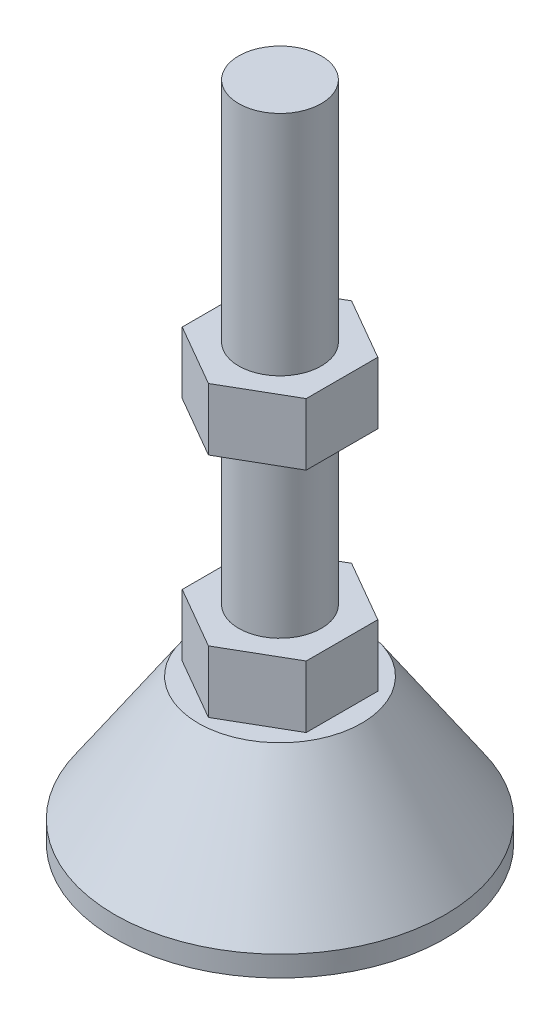
SolidWorks part; units mm, degrees
ref_plane "前视基准面" through (0, 0, 0) normal (0, 0, 1) x (1, 0, 0)
ref_plane "上视基准面" through (0, 0, 0) normal (0, 1, 0) x (1, 0, 0)
ref_plane "右视基准面" through (0, 0, 0) normal (1, 0, 0) x (0, 0, -1)
sketch "草图1" plane through (0, 0, 0) normal (0, 1, 0) x (1, 0, 0)
  circle A0 centre (0, 0) radius 40
  dimension "D1" = 80
extrude "凸台-拉伸1" add sketch "草图1" along normal blind 30 draft 34
sketch "草图2" plane through (0, 30, 0) normal (0, 1, 0) x (1, 0, 0)
  circle A0 centre (0, 0) radius 10
  dimension "D1" = 20
extrude "凸台-拉伸2" add sketch "草图2" along normal blind 125
sketch "草图3" plane through (0, 30, 0) normal (0, 1, 0) x (1, 0, 0)
  line L1 (15, -8.6603) -> (15, 8.6603)
  line L2 (15, 8.6603) -> (0, 17.3205)
  line L3 (0, 17.3205) -> (-15, 8.6603)
  line L4 (-15, 8.6603) -> (-15, -8.6603)
  line L5 (-15, -8.6603) -> (0, -17.3205)
  line L6 (0, -17.3205) -> (15, -8.6603)
  circle A0 centre (0, 0) radius 15 construction
  dimension "D1" = 30
extrude "凸台-拉伸3" add sketch "草图3" along normal blind 15
sketch "草图4" plane through (0, 0, 0) normal (0, -1, 0) x (1, 0, 0)
  circle A1 centre (0, 0) radius 40
  circle A2 centre (0, 0) radius 40
  dimension "D1" = 0
extrude "凸台-拉伸4" add sketch "草图4" along normal blind 5
sketch "草图5" plane through (0, 45, 0) normal (0, 1, 0) x (1, 0, 0)
  line L6 (0, -17.3205) -> (15, -8.6603)
  line L7 (15, -8.6603) -> (15, 8.6603)
  line L8 (15, 8.6603) -> (0, 17.3205)
  line L9 (0, 17.3205) -> (-15, 8.6603)
  line L10 (-15, 8.6603) -> (-15, -8.6603)
  line L11 (-15, -8.6603) -> (0, -17.3205)
  line L12 (0, -17.3205) -> (15, -8.6603)
  line L13 (15, -8.6603) -> (15, 8.6603)
  line L14 (15, 8.6603) -> (0, 17.3205)
  line L15 (0, 17.3205) -> (-15, 8.6603)
  line L16 (-15, 8.6603) -> (-15, -8.6603)
  line L17 (-15, -8.6603) -> (0, -17.3205)
  dimension "D1" = 0
extrude "凸台-拉伸5" add sketch "草图5" along normal blind 15 from offset 40
